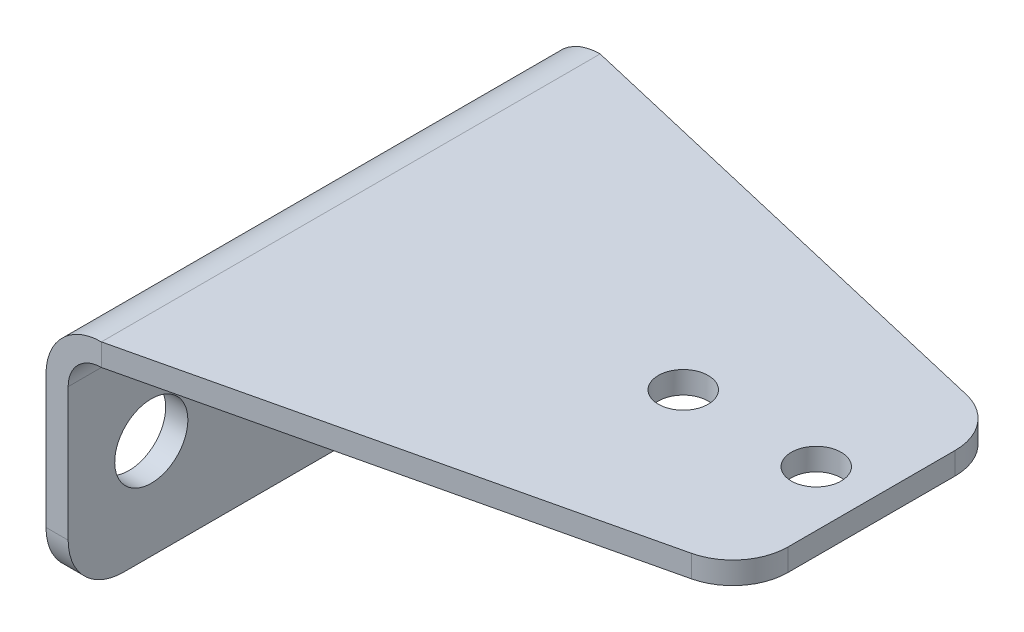
SolidWorks part; units mm, degrees
material "Stainless steel"
ref_plane "Front Plane" through (0, 0, 0) normal (0, 0, 1) x (1, 0, 0)
ref_plane "Top Plane" through (0, 0, 0) normal (0, 1, 0) x (1, 0, 0)
ref_plane "Right Plane" through (0, 0, 0) normal (1, 0, 0) x (0, 0, -1)
sketch "Sketch1" plane through (0, 0, 0) normal (0, 0, 1) x (1, 0, 0)
  line L0 (0, 0) -> (0, 17)
  line L1 (5, 22) -> (52, 22)
  line L2 (52, 22) -> (52, 20)
  line L3 (52, 20) -> (5, 20)
  line L4 (2, 17) -> (2, 0)
  line L5 (2, 0) -> (0, 0)
  arc A0 (0, 17) -> (5, 22) centre (5, 17) cw
  arc A1 (5, 20) -> (2, 17) centre (5, 17) ccw
  dimension "D3" = 5
  dimension "D4" = 3
  dimension "D1" = 2
  dimension "D2" = 2
  dimension "D5" = 20
  dimension "D6" = 52
extrude "Boss-Extrude1" add sketch "Sketch1" along normal blind 45
sketch "Sketch2" plane through (2, 0, 0) normal (1, 0, 0) x (0, 0, -1)
  line L0 (-45, 20) -> (0, 20) construction
  line L1 (-45, 0) -> (-45, 17) construction
  line L2 (0, 0) -> (0, 17) construction
  circle A0 centre (-37.5, 9) radius 3.3
  circle A1 centre (-7.5, 9) radius 3.3
  dimension "D1" = 11
  dimension "D2" = 6.6
  dimension "D3" = 30
  dimension "D5" = 7.5
  dimension "D4" = 7.5
extrude "Cut-Extrude1" cut sketch "Sketch2" against normal up to next
sketch "Sketch3" plane through (0, 22, 0) normal (0, 1, 0) x (1, 0, 0)
  line L0 (0, -45) -> (0, 0) construction
  line L1 (52, 0) -> (5, 0) construction
  line L2 (52, -45) -> (5, -45) construction
  circle A0 centre (35, -22.5) radius 2.25
  circle A1 centre (47, -22.5) radius 2.25
  dimension "D2" = 12
  dimension "D3" = 4.5
  dimension "D5" = 22.5
  dimension "D1" = 35
  dimension "D4" = 22.5
extrude "Cut-Extrude2" cut sketch "Sketch3" against normal up to next
sketch "Sketch4" plane through (0, 22, 0) normal (0, 1, 0) x (1, 0, 0)
  line L0 (5, 0) -> (52, -11)
  line L1 (52, -45) -> (52, 0) construction
  line L2 (52, -11) -> (52, 0)
  line L3 (52, 0) -> (5, 0)
  line L4 (52, 0) -> (5, 0) construction
  line L5 (5, -45) -> (52, -34)
  line L6 (52, -34) -> (52, -45)
  line L7 (52, -45) -> (5, -45)
  dimension "D1" = 23
extrude "Cut-Extrude3" cut sketch "Sketch4" against normal up to next
fillet "Fillet1" radius 5 4 edges at (1, 0, 0) (1, 0, 45) (52, 21, 11) (52, 21, 34)
